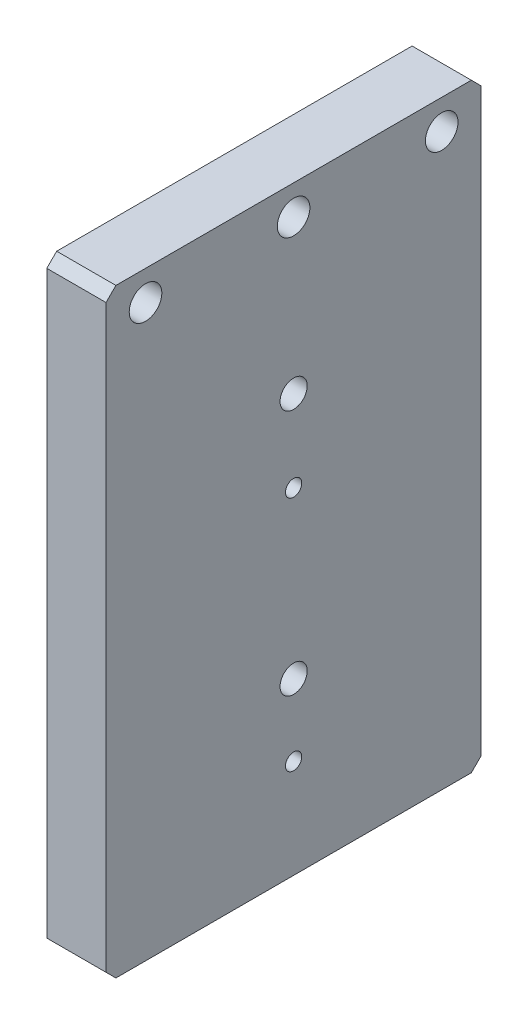
from build123d import *

# Parameters (mm, degrees)
SKETCH_1_W                   = 76
SKETCH_1_H                   = 121.5
EXTRUDE_1_DEPTH              = 12
HOLE_WIZARD_M6_1_D           = 6.6
HOLE_WIZARD_M6_1_CBORE_D     = 11
HOLE_WIZARD_M6_1_CBORE_DEPTH = 6.8
HOLE_WIZARD_M4_1_D           = 3.3
F_5_0MM_1_D                  = 5
F_5_0MM_1_DEPTH              = 6
F_5_0MM_1_TIP                = 1.502151548
HOLE_WIZARD_M5_1_D           = 5.5
HOLE_WIZARD_M5_1_DEPTH       = 12.4
HOLE_WIZARD_M5_1_CBORE_D     = 10
HOLE_WIZARD_M5_1_CBORE_DEPTH = 5.7
HOLE_WIZARD_M5_1_TIP         = 1.652366702
CHAMFER_1_SIZE               = 2


with BuildPart() as part:
    # 草图1 → 凸台-拉伸1 (new body)
    with BuildSketch(Plane(origin=(0, 0, 0), x_dir=(0, 0, -1), z_dir=(1, 0, 0))):
        Rectangle(SKETCH_1_W, SKETCH_1_H)
    extrude(amount=EXTRUDE_1_DEPTH)

    # M6 六角圆柱头螺钉的柱形沉头孔1 (through all)
    with Locations(Plane.ZY):
        with Locations((30, 54.75), (-30, 54.75), (0, 54.75)):
            CounterBoreHole(HOLE_WIZARD_M6_1_D / 2, HOLE_WIZARD_M6_1_CBORE_D / 2, HOLE_WIZARD_M6_1_CBORE_DEPTH)

    # M4 螺纹孔1 (through all)
    with Locations(Plane.ZY):
        with Locations((0, 7.25), (0, -40.75)):
            Hole(HOLE_WIZARD_M4_1_D / 2)

    # Ø5.0mm 暗销孔1
    with Locations(Plane.ZY):
        with Locations((24, 7.25), (24, -40.75), (-24, -40.75), (-24, 7.25)):
            Hole(F_5_0MM_1_D / 2, depth=F_5_0MM_1_DEPTH)
            with Locations((0, 0, -(F_5_0MM_1_DEPTH + F_5_0MM_1_TIP / 2))):  # 118° drill point
                Cone(0, F_5_0MM_1_D / 2, F_5_0MM_1_TIP, mode=Mode.SUBTRACT)

    # M5 六角圆柱头螺钉的柱形沉头孔1
    with Locations(Plane.ZY):
        with Locations((0, 23.75), (0, -26.25)):
            CounterBoreHole(HOLE_WIZARD_M5_1_D / 2, HOLE_WIZARD_M5_1_CBORE_D / 2, HOLE_WIZARD_M5_1_CBORE_DEPTH, depth=HOLE_WIZARD_M5_1_DEPTH)
            with Locations((0, 0, -(HOLE_WIZARD_M5_1_DEPTH + HOLE_WIZARD_M5_1_TIP / 2))):  # 118° drill point
                Cone(0, HOLE_WIZARD_M5_1_D / 2, HOLE_WIZARD_M5_1_TIP, mode=Mode.SUBTRACT)

    # 倒角1
    chamfer_1_edges = [part.edges().sort_by_distance(p)[0] for p in [
        (6, -60.75, -38),
        (6, -60.75, 38),
        (6, 60.75, 38),
        (6, 60.75, -38),
    ]]
    chamfer(chamfer_1_edges, length=CHAMFER_1_SIZE)


solid = part.part
